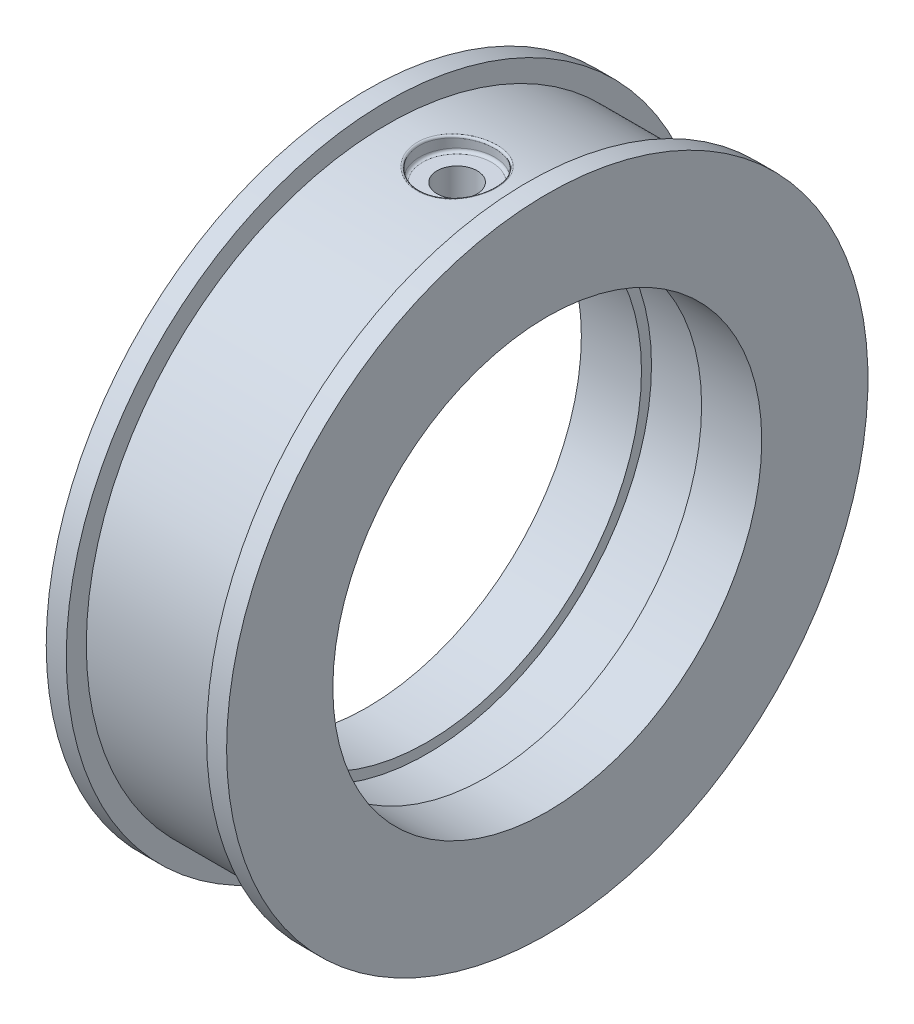
SolidWorks part; units mm, degrees
ref_plane "Front Plane" through (0, 0, 0) normal (0, 0, 1) x (1, 0, 0)
ref_plane "Top Plane" through (0, 0, 0) normal (0, 1, 0) x (1, 0, 0)
ref_plane "Right Plane" through (0, 0, 0) normal (1, 0, 0) x (0, 0, -1)
sketch "Sketch1" plane through (0, 0, 0) normal (0, 0, 1) x (1, 0, 0)
  line L0 (-19.0368, 0) -> (19.2228, 0) construction
  line L1 (-8.3897, 21.4) -> (-8.3897, 32)
  line L2 (-8.3897, 32) -> (-6.3897, 32)
  line L3 (-6.3897, 32) -> (-6.3897, 30)
  line L4 (-6.3897, 30) -> (7.6103, 30)
  line L5 (7.6103, 30) -> (7.6103, 32)
  line L6 (7.6103, 32) -> (9.6103, 32)
  line L7 (9.6103, 32) -> (9.6103, 21.4)
  line L8 (9.6103, 21.4) -> (3.6103, 21.4)
  line L9 (3.6103, 21.4) -> (3.6103, 22.4)
  line L10 (3.6103, 22.4) -> (-2.3897, 22.4)
  line L11 (-2.3897, 22.4) -> (-2.3897, 21.4)
  line L12 (-2.3897, 21.4) -> (-8.3897, 21.4)
  dimension "D2" = 18
  dimension "D3" = 14
  dimension "D4" = 2
  dimension "D5" = 21.4
  dimension "D6" = 21.4
  dimension "D7" = 22.4
  dimension "D8" = 6
  dimension "D9" = 6
  dimension "D10" = 30
  dimension "D11" = 32
  dimension "D12" = 32
revolve "Revolve1" add sketch "Sketch1" angle 360 about L0
ref_plane "Plane1" through (0, 30, 0) normal (0, 1, 0) x (1, 0, 0)
sketch "Sketch2" plane through (0, 30, 0) normal (0, 1, 0) x (1, 0, 0)
  line L0 (-6.3897, 0) -> (7.6103, 0)
  line L1 (-6.3897, -32) -> (-6.3897, 32) construction
  line L2 (7.6103, 30) -> (7.6103, -30) construction
hole_wizard "Hole1" positions "Sketch3" profile "Sketch4" legacy
sketch "Sketch3" plane through (0, 30, 0) normal (0, 1, 0) x (1, 0, 0)
  line L0 (-6.3897, 0) -> (7.6103, 0) construction
  point P0 (0.6103, 0)
sketch "Sketch4" plane through (0.6103, 30, 0) normal (1, 0, 0) x (0, 0, 1)
  line L0 (0, 0) -> (0, 1.5)
  line L1 (0, 1.5) -> (3.75, 1.5)
  line L2 (3.75, 1.5) -> (3.75, 0)
  line L3 (3.75, 0) -> (0, 0)
  line L4 (0, 110) -> (0, -10) construction
  dimension "直径" = 7.5
  dimension "深度" = 1.5
hole_wizard "Hole2" positions "Sketch5" profile "Sketch6" legacy
sketch "Sketch5" plane through (0, 28.5, 0) normal (0, 1, 0) x (1, 0, 0)
  point P0 (0.6103, 0)
sketch "Sketch6" plane through (0.6103, 28.5, 0) normal (1, 0, 0) x (0, 0, 1)
  line L0 (0, 0) -> (0, 6.1)
  line L1 (0, 6.1) -> (2, 6.1)
  line L2 (2, 6.1) -> (2, 0)
  line L3 (2, 0) -> (0, 0)
  line L4 (0, 110) -> (0, -10) construction
  dimension "直径" = 4
  dimension "深度" = 6.1
ref_plane "Plane2" through (0, -30, 0) normal (0, -1, 0) x (-1, 0, 0)
sketch "Sketch8" plane through (0, -30, 0) normal (0, -1, 0) x (-1, 0, 0)
  line L0 (6.3897, 0) -> (-7.6103, 0) construction
  line L1 (6.3897, 0) -> (-7.6103, 0)
hole_wizard "Dowel Hole1" positions "Sketch9" profile "Sketch10" hole size "Ø4.0" standard "GB"
sketch "Sketch9" plane through (0, -30, 0) normal (0, -1, 0) x (-1, 0, 0)
  line L0 (6.3897, 0) -> (-7.6103, 0) construction
  point P0 (-0.6103, 0)
sketch "Sketch10" plane through (0.6103, -30, 0) normal (1, 0, 0) x (0, 0, -1)
  line L0 (0, 0) -> (0, 5.2017)
  line L1 (0, 5.2017) -> (2, 4)
  line L2 (2, 4) -> (2, 0)
  line L5 (2, 0) -> (0, 0)
  line L10 (0, 5.2017) -> (-2, 4) construction
  line L11 (0, -6.35) -> (0, 107.95) construction
  dimension "孔直径" = 4
  dimension "孔深度" = 4
  dimension "导头角度" = 118
fillet "Fillet1" radius 0.2 1 edges at (1.44, 29.7763, -3.6571)
fillet "Fillet2" radius 0.3 1 edges at (0.6103, 28.5, 3.75)
